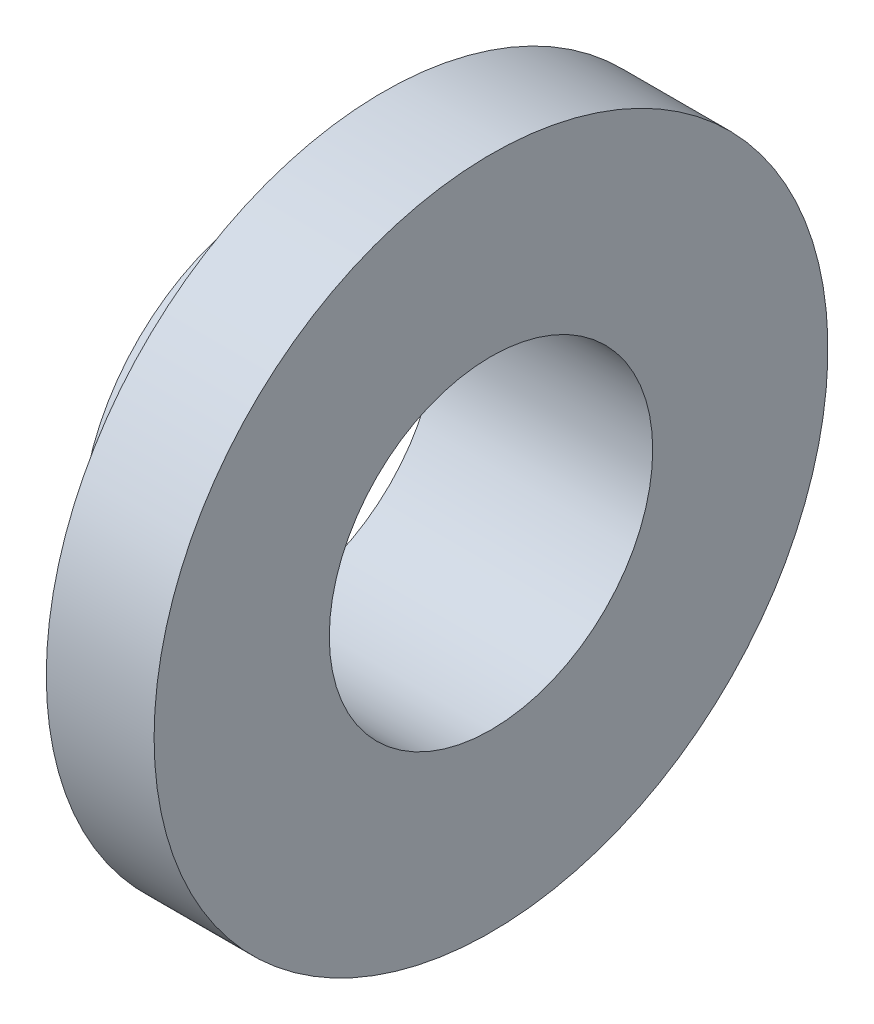
SolidWorks part; units mm, degrees
material "35"
ref_plane "Front Plane" through (0, 0, 0) normal (0, 0, 1) x (1, 0, 0)
ref_plane "Top Plane" through (0, 0, 0) normal (0, 1, 0) x (1, 0, 0)
ref_plane "Right Plane" through (0, 0, 0) normal (1, 0, 0) x (0, 0, -1)
sketch "Sketch1" plane through (0, 0, 0) normal (0, 0, 1) x (1, 0, 0)
  line L0 (0, 0) -> (78.9231, 0) construction
  line L1 (0, -30) -> (0, -36)
  line L2 (0, -36) -> (20, -36)
  line L3 (20, -36) -> (20, -62.5)
  line L4 (20, -62.5) -> (40, -62.5)
  line L5 (40, -62.5) -> (40, -30)
  line L6 (40, -30) -> (0, -30)
  dimension "D1" = 30
  dimension "D2" = 36
  dimension "D3" = 62.5
  dimension "D4" = 40
  dimension "D5" = 20
revolve "Revolve1" add sketch "Sketch1" angle 360 about L0
